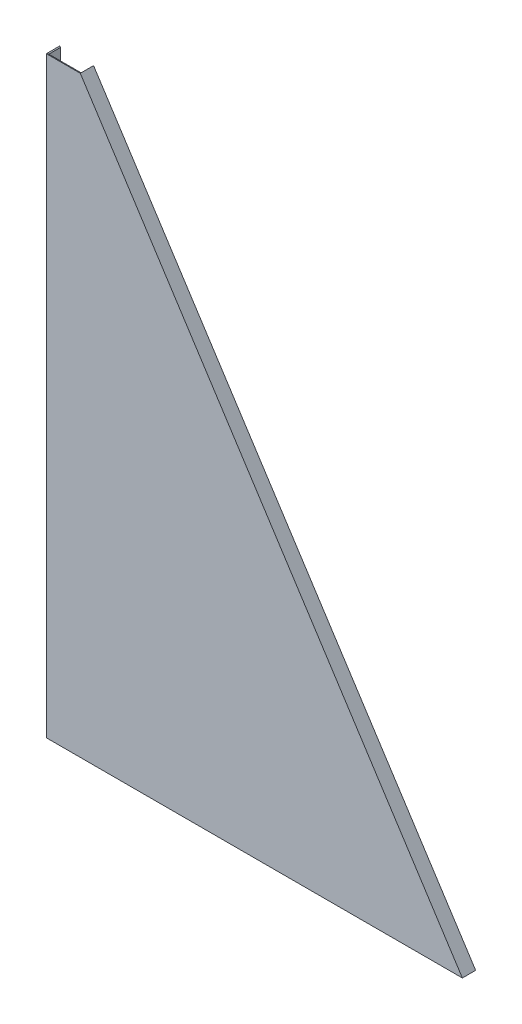
SolidWorks part; units mm, degrees
material "1023 碳钢板 (SS)"
ref_plane "Front Plane" through (0, 0, 0) normal (0, 0, 1) x (1, 0, 0)
ref_plane "Top Plane" through (0, 0, 0) normal (0, 1, 0) x (1, 0, 0)
ref_plane "Right Plane" through (0, 0, 0) normal (1, 0, 0) x (0, 0, -1)
sketch "Sketch1" plane through (0, 0, 0) normal (0, 0, 1) x (1, 0, 0)
  line L1 (-501, 713.5) -> (501, 713.5)
  line L2 (-501, 713.5) -> (-501, -713.5)
  line L3 (-501, -713.5) -> (501, -713.5)
  line L4 (501, 713.5) -> (501, -713.5)
  line L5 (-501, 713.5) -> (501, -713.5) construction
  line L6 (-501, -713.5) -> (501, 713.5) construction
  point P0 (0, 0)
  dimension "D1" = 1002
  dimension "D2" = 1427
extrude "Boss-Extrude1" add sketch "Sketch1" along normal blind 2
sketch "Sketch2" plane through (0, 0, 2) normal (0, 0, 1) x (1, 0, 0)
  line L0 (-419.25, 713.5) -> (501, -713.5)
  line L2 (501, -713.5) -> (501, 713.5) construction
  line L3 (-419.25, 713.5) -> (501, 713.5)
  line L4 (501, 713.5) -> (501, -713.5)
  line L5 (-501, -713.5) -> (501, -713.5) construction
  dimension "D1" = 1427
  dimension "D2" = 920.25
extrude "Cut-Extrude1" cut sketch "Sketch2" against normal blind 2
sketch "Sketch4" plane through (0, 0, 0) normal (0, 0, -1) x (-1, 0, 0)
  line L0 (420.34, 711.5) -> (-497.3304, -711.5)
  line L1 (-497.3304, -711.5) -> (499, -711.5)
  line L2 (499, -711.5) -> (499, 711.5)
  line L4 (501, 713.5) -> (419.25, 713.5)
  line L5 (419.25, 713.5) -> (-501, -713.5)
  line L6 (-501, -713.5) -> (501, -713.5)
  line L7 (501, -713.5) -> (501, 713.5)
  line L9 (419.25, 713.5) -> (-501, -713.5)
  line L10 (-501, -713.5) -> (501, -713.5)
  line L11 (501, -713.5) -> (501, 713.5)
  line L12 (419.25, 713.5) -> (420.34, 711.5)
  line L13 (501, 713.5) -> (499, 711.5)
  line L16 (501, 713.5) -> (419.25, 713.5) construction
  line L17 (499, 711.5) -> (420.34, 711.5) construction
  dimension "D1" = 0
  dimension "D2" = 2
extrude "Boss-Extrude2" add sketch "Sketch4" along normal blind 30
